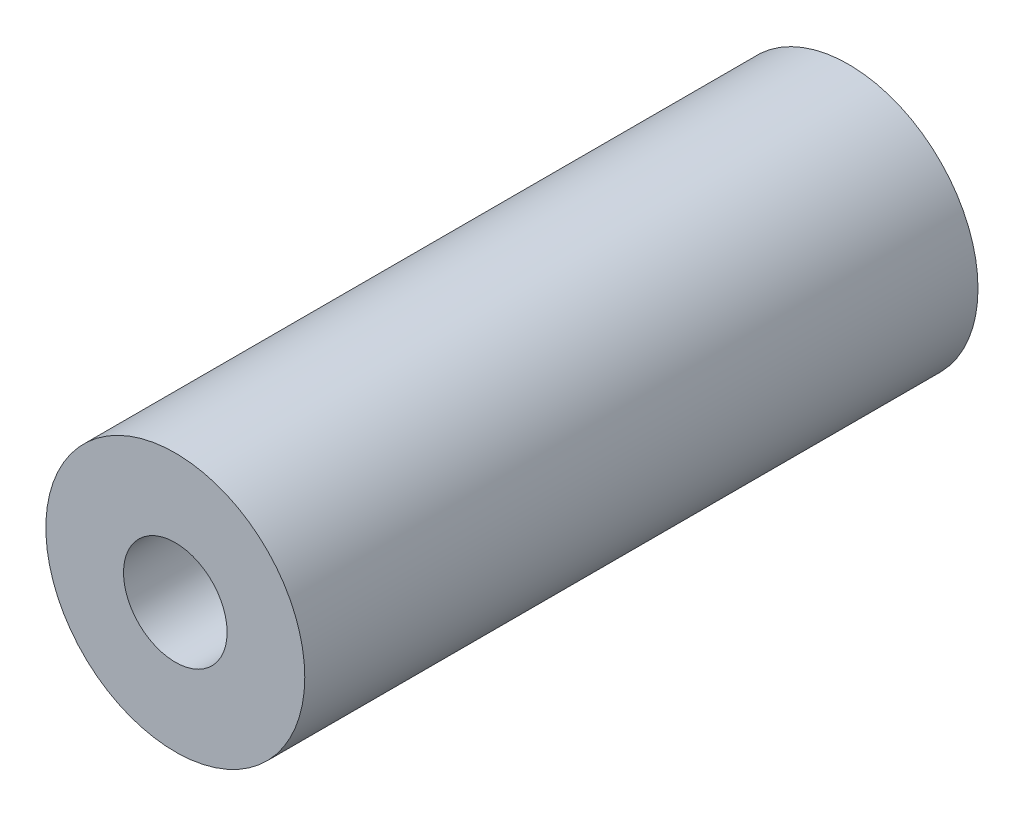
SolidWorks part; units mm, degrees
ref_plane "前视基准面" through (0, 0, 0) normal (0, 0, 1) x (1, 0, 0)
ref_plane "上视基准面" through (0, 0, 0) normal (0, 1, 0) x (1, 0, 0)
ref_plane "右视基准面" through (0, 0, 0) normal (1, 0, 0) x (0, 0, -1)
other "Configuration Table"
sketch "草图1" plane through (0, 0, 0) normal (0, 0, 1) x (1, 0, 0)
  circle A0 centre (0, 0) radius 5
  circle A1 centre (0, 0) radius 2
  point P0 (0, 0)
  dimension "D1" = 4
  dimension "D2" = 10
extrude "凸台-拉伸1" add sketch "草图1" against normal mid plane 26
